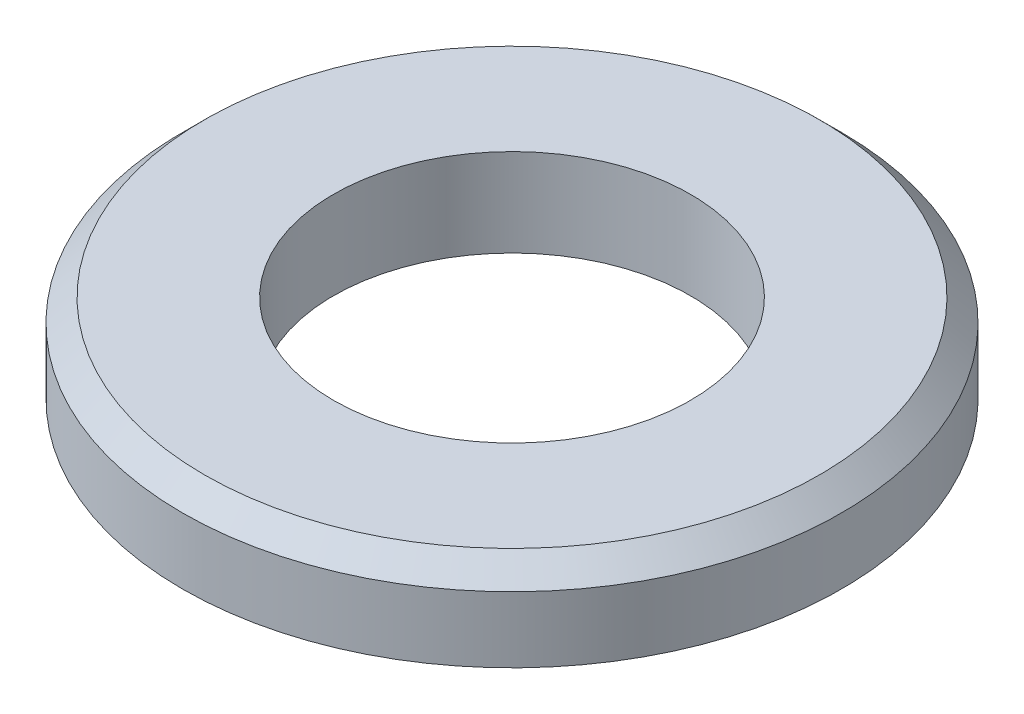
SolidWorks part; units mm, degrees
ref_plane "Front Plane" through (0, 0, 0) normal (0, 0, 1) x (1, 0, 0)
ref_plane "Top Plane" through (0, 0, 0) normal (0, 1, 0) x (1, 0, 0)
ref_plane "Right Plane" through (0, 0, 0) normal (1, 0, 0) x (0, 0, -1)
sketch "Sketch1" plane through (0, 0, 0) normal (0, 1, 0) x (1, 0, 0)
  circle A0 centre (0, 0) radius 6
  circle A1 centre (0, 0) radius 3.25
  dimension "D1" = 12
  dimension "D2" = 6.5
extrude "Boss-Extrude1" add sketch "Sketch1" along normal blind 1.6
chamfer "Chamfer1" distance 0.4 angle 45 1 edges at (0, 1.6, 6)
